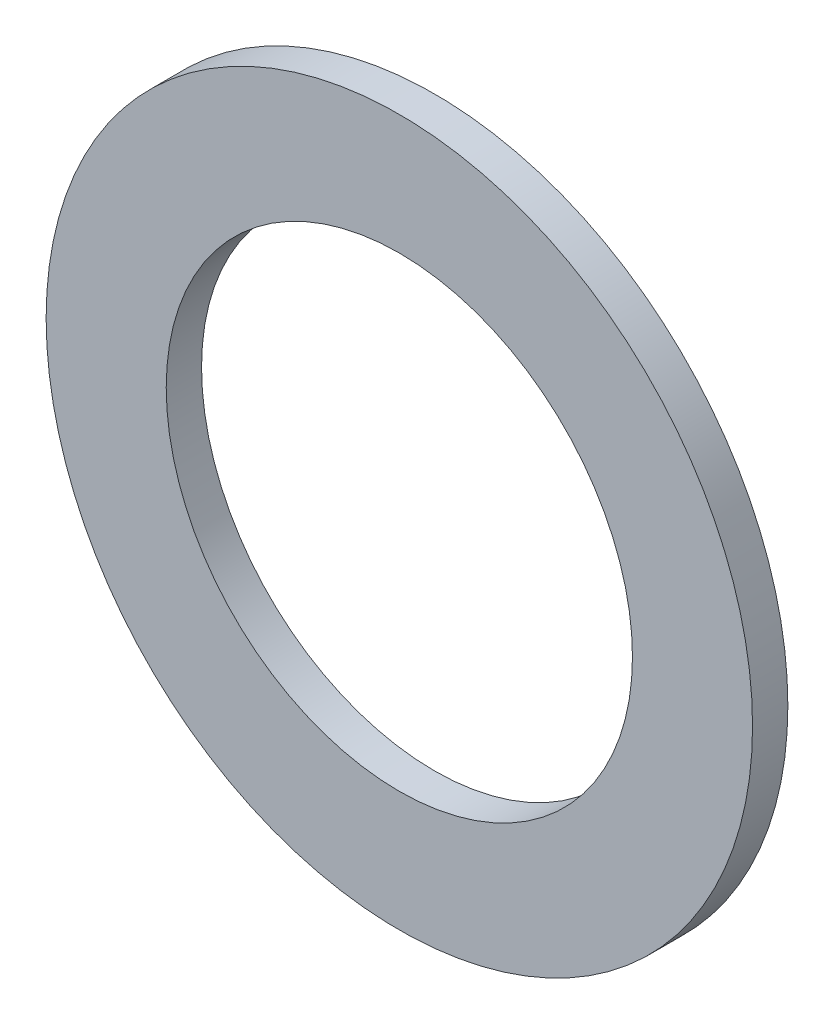
from build123d import *

# Parameters (mm, degrees)
SKETCH_1_R      = 50
SKETCH_1_R_2    = 33
EXTRUDE_1_DEPTH = 5


with BuildPart() as part:
    # 草图1 → 凸台-拉伸1 (new body)
    with BuildSketch(Plane.XY):
        Circle(SKETCH_1_R)
        Circle(SKETCH_1_R_2, mode=Mode.SUBTRACT)
    extrude(amount=EXTRUDE_1_DEPTH)


solid = part.part
